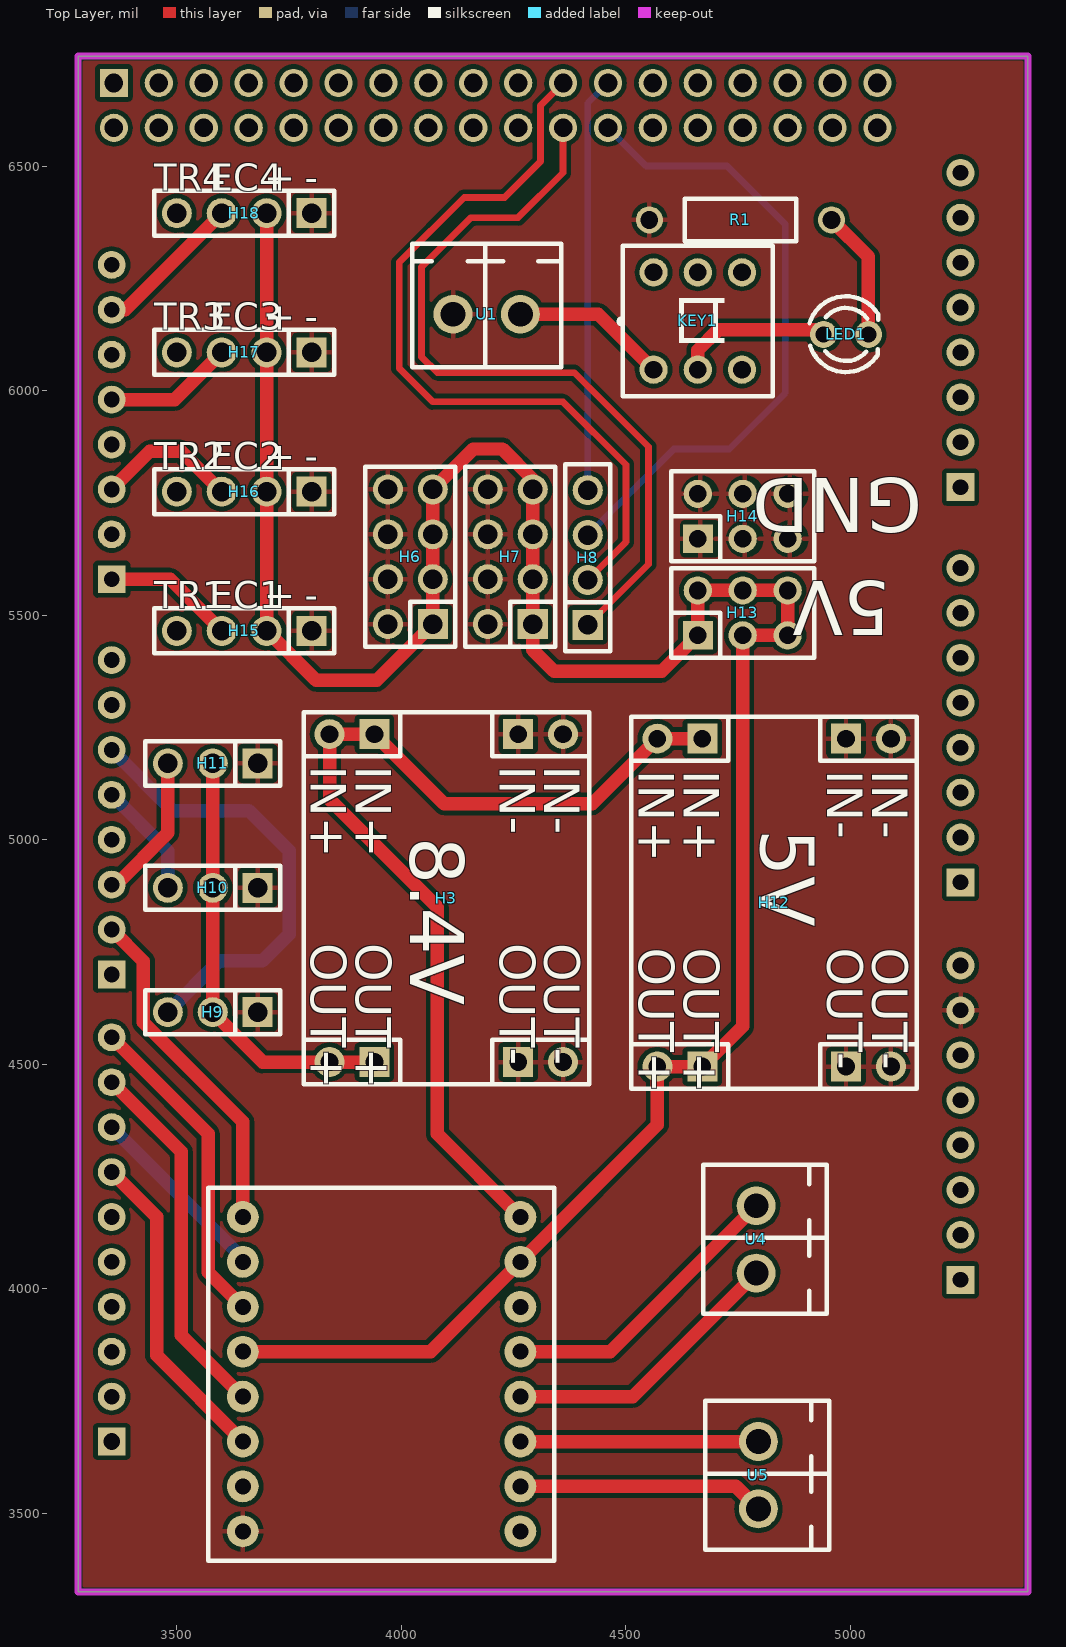
[diagram p0: Top Layer view]
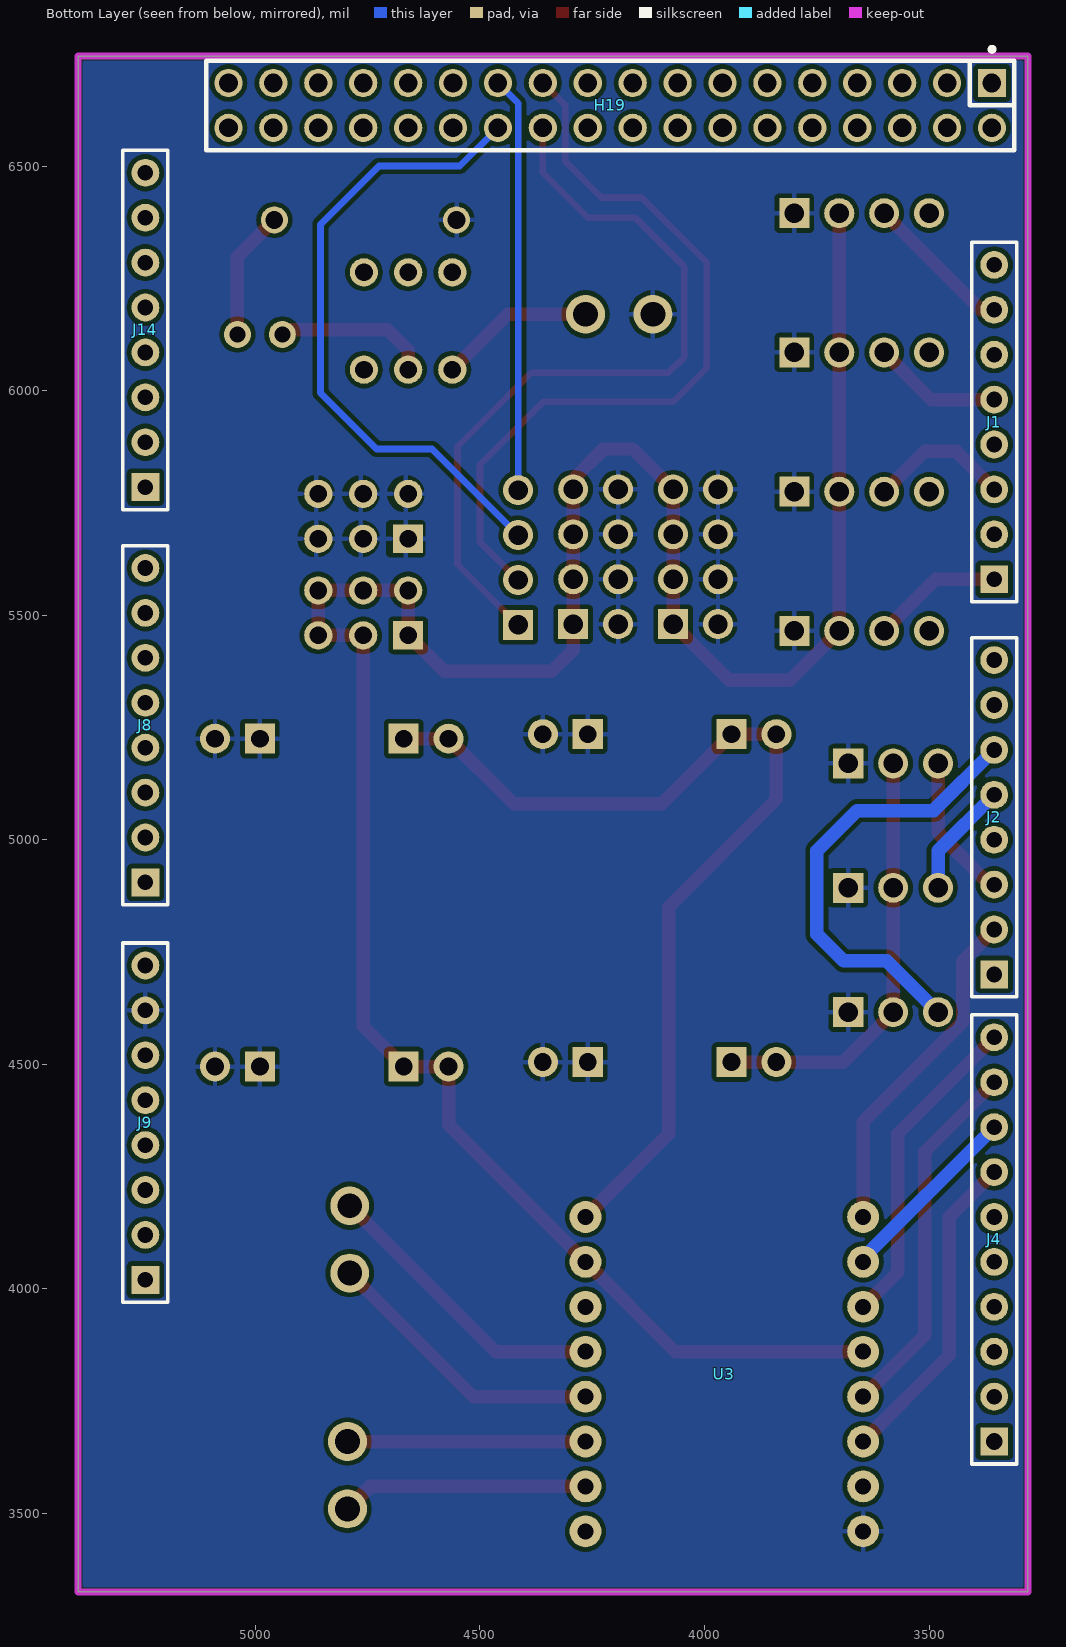
[diagram p1: Bottom Layer view, seen from below]
# Altium PCB MISC49940.pcbdoc
Units mil, origin at the board's own origin, x right, y up, seen from the top; angles counter-clockwise.
Board outline 2115 x 3420 mil, 2 copper layers (Top Layer, Bottom Layer), stack 62.206 mil thick; 28 components, 38 nets, 191 pads, 0 vias.

## Layer stack, top to bottom
Top Solder Mask Layer: solder mask 0.394, Dk 3.3
Top Layer: signal copper 1.379
Dielectric1: surface 59.449, FR4, Dk 4.5
Bottom Layer: signal copper 1.378
Bottom Solder Mask Layer: solder mask 0.394, Dk 3.3

## Board outline
3280,6745 3280,3325 5395,3325 5395,6745

## Design rules (kind name [scope] priority, off if disabled: settings)
BoardOutlineClearance copperThickness2oz_1 [All] p2 off: genericclearance=7.99 ignorepadtopadclearanceinfootprint=FALSE except(0: Arc-SplitContinuation Track-SplitContinuation SMDPad-SplitContinuation THPad-SplitContinuation Via-SplitContinuation Fill-SplitContinuation Region-SplitContinuation Poly-SplitContinuation Text-SplitContinuation Hole-SplitContinuation; 5.98: Arc-CutoutEdge Track-CutoutEdge SMDPad-CutoutEdge THPad-CutoutEdge Via-CutoutEdge Text-CutoutEdge; 6.9: Hole-OutlineEdge Hole-CutoutEdge; 10: Poly-OutlineEdge Poly-CutoutEdge; 11.81: Arc-OutlineEdge Track-OutlineEdge SMDPad-OutlineEdge THPad-OutlineEdge Via-OutlineEdge Fill-OutlineEdge Region-OutlineEdge Text-OutlineEdge Fill-CutoutEdge Region-CutoutEdge)
BoardOutlineClearance Plane_innerPlane_1 [All] p4 off: genericclearance=4.02 ignorepadtopadclearanceinfootprint=FALSE except(0: Arc-SplitContinuation Track-SplitContinuation SMDPad-SplitContinuation THPad-SplitContinuation Via-SplitContinuation Fill-SplitContinuation Region-SplitContinuation Poly-SplitContinuation Text-SplitContinuation Hole-SplitContinuation; 5.98: Arc-CutoutEdge Track-CutoutEdge SMDPad-CutoutEdge THPad-CutoutEdge Via-CutoutEdge Text-CutoutEdge; 6.9: Hole-OutlineEdge Hole-CutoutEdge; 10: Poly-OutlineEdge Poly-CutoutEdge; 11.81: Arc-OutlineEdge Track-OutlineEdge SMDPad-OutlineEdge THPad-OutlineEdge Via-OutlineEdge Fill-OutlineEdge Region-OutlineEdge Text-OutlineEdge Fill-CutoutEdge Region-CutoutEdge)
BoardOutlineClearance Copper_copperRegion_1 [All] p6 off: genericclearance=4.02 ignorepadtopadclearanceinfootprint=FALSE except(0: Arc-SplitContinuation Track-SplitContinuation SMDPad-SplitContinuation THPad-SplitContinuation Via-SplitContinuation Fill-SplitContinuation Region-SplitContinuation Poly-SplitContinuation Text-SplitContinuation Hole-SplitContinuation; 5.98: Arc-CutoutEdge Track-CutoutEdge SMDPad-CutoutEdge THPad-CutoutEdge Via-CutoutEdge Text-CutoutEdge; 6.9: Hole-OutlineEdge Hole-CutoutEdge; 10: Poly-OutlineEdge Poly-CutoutEdge; 11.81: Arc-OutlineEdge Track-OutlineEdge SMDPad-OutlineEdge THPad-OutlineEdge Via-OutlineEdge Fill-OutlineEdge Region-OutlineEdge Text-OutlineEdge Fill-CutoutEdge Region-CutoutEdge)
BoardOutlineClearance copperThickness1oz_1 [All] p8: genericclearance=4.02 ignorepadtopadclearanceinfootprint=FALSE except(0: Arc-SplitContinuation Track-SplitContinuation SMDPad-SplitContinuation THPad-SplitContinuation Via-SplitContinuation Fill-SplitContinuation Region-SplitContinuation Poly-SplitContinuation Text-SplitContinuation Hole-SplitContinuation; 5.98: Arc-CutoutEdge Track-CutoutEdge SMDPad-CutoutEdge THPad-CutoutEdge Via-CutoutEdge Text-CutoutEdge; 6.9: Hole-OutlineEdge Hole-CutoutEdge; 10: Poly-OutlineEdge Poly-CutoutEdge; 11.81: Arc-OutlineEdge Track-OutlineEdge SMDPad-OutlineEdge THPad-OutlineEdge Via-OutlineEdge Fill-OutlineEdge Region-OutlineEdge Text-OutlineEdge Fill-CutoutEdge Region-CutoutEdge)
Clearance copperThickness2oz [All] p1 off: gap=7.99 ignorepadtopadclearanceinfootprint=FALSE except(5.98: SMDPad-Track SMDPad-SMDPad THPad-Track SMDPad-THPad THPad-THPad Track-Via SMDPad-Via THPad-Via Via-Via Fill-SMDPad Region-SMDPad Fill-THPad Region-THPad Fill-Via Region-Via Fill-Fill Fill-Region Region-Region Arc-Track Arc-SMDPad Arc-THPad Arc-Via Fill-Arc Region-Arc Arc-Arc Text-Track SMDPad-Text Text-THPad Text-Via Fill-Text Region-Text Arc-Text Text-Text; 6.9: Hole-Track Hole-SMDPad Hole-THPad Hole-Via Fill-Hole Region-Hole Hole-Arc Hole-Text; 10: Poly-Track Poly-SMDPad Poly-THPad Poly-Via Poly-Fill Poly-Region Poly-Poly Poly-Arc Poly-Text Poly-Hole; 11.81: Fill-Track Region-Track)
Clearance Plane_innerPlane [All] p3 off: gap=4.02 ignorepadtopadclearanceinfootprint=FALSE except(5.98: SMDPad-Track SMDPad-SMDPad THPad-Track SMDPad-THPad THPad-THPad Track-Via SMDPad-Via THPad-Via Via-Via Fill-SMDPad Region-SMDPad Fill-THPad Region-THPad Fill-Via Region-Via Fill-Fill Fill-Region Region-Region Arc-Track Arc-SMDPad Arc-THPad Arc-Via Fill-Arc Region-Arc Arc-Arc Text-Track SMDPad-Text Text-THPad Text-Via Fill-Text Region-Text Arc-Text Text-Text; 6.9: Hole-Track Hole-SMDPad Hole-THPad Hole-Via Fill-Hole Region-Hole Hole-Arc Hole-Text; 10: Poly-Track Poly-SMDPad Poly-THPad Poly-Via Poly-Fill Poly-Region Poly-Poly Poly-Arc Poly-Text Poly-Hole; 11.81: Fill-Track Region-Track)
Clearance Copper_copperRegion [All] p5 off: gap=4.02 ignorepadtopadclearanceinfootprint=FALSE except(5.98: SMDPad-Track SMDPad-SMDPad THPad-Track SMDPad-THPad THPad-THPad Track-Via SMDPad-Via THPad-Via Via-Via Fill-SMDPad Region-SMDPad Fill-THPad Region-THPad Fill-Via Region-Via Fill-Fill Fill-Region Region-Region Arc-Track Arc-SMDPad Arc-THPad Arc-Via Fill-Arc Region-Arc Arc-Arc Text-Track SMDPad-Text Text-THPad Text-Via Fill-Text Region-Text Arc-Text Text-Text; 6.9: Hole-Track Hole-SMDPad Hole-THPad Hole-Via Fill-Hole Region-Hole Hole-Arc Hole-Text; 10: Poly-Track Poly-SMDPad Poly-THPad Poly-Via Poly-Fill Poly-Region Poly-Poly Poly-Arc Poly-Text Poly-Hole; 11.81: Fill-Track Region-Track)
Clearance copperThickness1oz [All] p7: gap=4.02 ignorepadtopadclearanceinfootprint=FALSE except(5.98: SMDPad-Track SMDPad-SMDPad THPad-Track SMDPad-THPad THPad-THPad Track-Via SMDPad-Via THPad-Via Via-Via Fill-SMDPad Region-SMDPad Fill-THPad Region-THPad Fill-Via Region-Via Fill-Fill Fill-Region Region-Region Arc-Track Arc-SMDPad Arc-THPad Arc-Via Fill-Arc Region-Arc Arc-Arc Text-Track SMDPad-Text Text-THPad Text-Via Fill-Text Region-Text Arc-Text Text-Text; 6.9: Hole-Track Hole-SMDPad Hole-THPad Hole-Via Fill-Hole Region-Hole Hole-Arc Hole-Text; 10: Poly-Track Poly-SMDPad Poly-THPad Poly-Via Poly-Fill Poly-Region Poly-Poly Poly-Arc Poly-Text Poly-Hole; 11.81: Fill-Track Region-Track)
DiffPairsRouting differentialPair [All] p1: maxlimit=6 minlimit=6 mostfreqgap=6 toplayer_minwidth=5 toplayer_prefwidth=10 toplayer_maxwidth=100 toplayer_mingap=6 toplayer_prefgap=6 toplayer_maxgap=6 bottomlayer_minwidth=5 bottomlayer_prefwidth=10 bottomlayer_maxwidth=100 bottomlayer_mingap=6 bottomlayer_prefgap=6 bottomlayer_maxgap=6 maxuncoupledlength=10
HoleToHoleClearance otherClearance [All] p1: gap=11.81 allowstackedmicrovias=TRUE
Length netLength [All] p1: minlimit=0 maxlimit=0
PasteMaskExpansion pasteMaskExpansion [All] p1: expansion=0
PlaneConnect innerPlane [All] p1: planeconnectstyle=Relief reliefexpansion=20 reliefentries=4 reliefconductorwidth=10 reliefairgap=10
PolygonConnect copperRegion [All] p1: connectstyle=Relief reliefconductorwidth=10 reliefentries=4 polygonreliefangle="90 Angle" airgapwidth=10 via.connectstyle=Relief via.reliefconductorwidth=10 via.reliefentries=4 via.polygonreliefangle="90 Angle" via.airgapwidth=10
RoutingVias viaSize [All] p1: holewidth=12.01 width=24.02 viastyle="Through Hole" minholewidth=11.81 minwidth=19.68 maxholewidth=248.03 maxwidth=393.7
SolderMaskExpansion solderMaskExpansion [IsVia] p1: expansion=-1000 istentingtop=TRUE
SolderMaskExpansion solderMaskExpansion [All] p2: expansion=2 istentingtop=FALSE
Width copperThickness2oz_2 [All] p1 off: maxlimit=100 minlimit=8 preferedwidth=10
Width copperThickness1oz_2 [All] p2: maxlimit=100 minlimit=5 preferedwidth=10

## Components (designator, comment, footprint, x,y, rotation, side; value= is the part's Value field where it differs from the comment)
H3 "" HDR-TH_8P-P2.54-V-M 4360,5235 r270 top
H6 "" HDR-TH_8P-P2.54-V-M-R2-C4-S2.54 4020,5630 r90 top
H7 "" HDR-TH_8P-P2.54-V-M-R2-C4-S2.54 4242.5,5630 r90 top
H8 "" HDR-TH_4P-P2.54-V-F 4415,5628.27 r90 top
H9 "" HDR-TH_3P-P2.54-V-M 3580,4616.01 r180 top
H10 "" HDR-TH_3P-P2.54-V-M 3580,4892.9 r180 top
H11 "" HDR-TH_3P-P2.54-V-M 3580,5169.79 r180 top
H12 "" HDR-TH_8P-P2.54-V-M 5090,5225 r270 top
H13 "" HDR-TH_6P-P2.54-V-F-R2-C3-S2.54 4760,5505 r0 top
H14 "" HDR-TH_6P-P2.54-V-F-R2-C3-S2.54 4760,5720 r0 top
H15 "" HDR-TH_4P-P2.54-V-M 3650,5465 r180 top
H16 "" HDR-TH_4P-P2.54-V-M 3650,5775 r180 top
H17 "" HDR-TH_4P-P2.54-V-M 3650,6085 r180 top
H18 "" HDR-TH_4P-P2.54-V-M 3650,6395 r180 top
H19 "X6521WV-2×18H-C30D60" HDR-TH_36P-2.54-V-M-R2-C18-S2.54 4210,6635 r0 bottom
J1 "3-way TX/RX" HDR-M-2.54_1X8 3355,5980 r90 bottom
J2 "PWM D2~D7" HDR-M-2.54_1X8 3355,5100 r90 bottom
J4 "PWM_D8~D13" HDR-M-2.54_1X10 3355,4110 r90 bottom
J8 "HDR-M-2.54_1x8" HDR-M-2.54_1X8 5245,5305 r90 bottom
J9 "HDR-M-2.54_1x8" HDR-M-2.54_1X8 5245,4420 r90 bottom
J14 "HDR-M-2.54_1x8" HDR-M-2.54_1X8 5245,6185 r90 bottom
KEY1 "Self-locking switch" SW-TH_6P-L8.5-W8.5-P2.54 4660,6155 r0 top
LED1 "" LED_TH-3mm 4990,6125 r0 top
R1 "1kΩ" Res_1/4W 4755,6380 r180 top
U1 "2P-P3.81_KF2EDGV-3.81-2P" CONN-TH_2P-P3.81_KF2EDGV-3.81-2P 4190,6170 r180 top
U3 "" tb6612 4265,4160 r180 bottom
U4 "2P-P3.81_KF2EDGV-3.81-2P" CONN-TH_2P-P3.81_KF2EDGV-3.81-2P 4790,4110 r90 top
U5 "2P-P3.81_KF2EDGV-3.81-2P" CONN-TH_2P-P3.81_KF2EDGV-3.81-2P 4795,3585 r90 top

## Footprints (in the part's own frame and the unit in brackets; to place one, negate y for a bottom-side part, rotate by r counter-clockwise, add the part's x,y. Pads: shape width x height; smd on the part's side, far side on the other; paste and mask are expansions set on the pad)
CONN-TH_2P-P3.81_KF2EDGV-3.81-2P [mm]
  round 2.2 hole 1.4: 1(-1.905,0) 2(1.905,0)
  silkscreen extent -4.21,-4 4.21,3
HDR-M-2.54_1X8 [mil]
  rect 62x62 hole 35: 1(-400,0)
  round 62 hole 35: 2(-300,0) 3(-200,0) 4(-100,0) 5(0,0) 6(100,0) 7(200,0) 8(300,0)
  silkscreen extent -450,-50 350,50
HDR-M-2.54_1X10 [mil]
  rect 62x62 hole 37.2: 1(-450,0)
  round 62 hole 35: 2(-350,0) 3(-250,0) 4(-150,0) 5(-50,0) 6(50,0) 7(150,0) 8(250,0) 9(350,0) 10(450,0)
  silkscreen extent -500,-50 500,50
HDR-TH_3P-P2.54-V-M [mm]
  rect 1.7x1.7 hole 1.1: 1(-2.54,0)
  round 1.7 hole 1.1: 2(0,0) 3(2.54,0)
  silkscreen extent -3.81,-1.25 3.81,1.25
HDR-TH_4P-P2.54-V-F [mm]
  rect 1.7x1.7 hole 1.1: 1(-3.81,0)
  round 1.7 hole 1.1: 2(-1.27,0) 3(1.27,0) 4(3.81,0)
  silkscreen extent -5.29,-1.27 5.29,1.27
HDR-TH_4P-P2.54-V-M [mm]
  rect 1.7x1.7 hole 1.1: 1(-3.81,0)
  round 1.7 hole 1.1: 2(-1.27,0) 3(1.27,0) 4(3.81,0)
  silkscreen extent -5.08,-1.27 5.08,1.27
HDR-TH_6P-P2.54-V-F-R2-C3-S2.54 [mm]
  rect 1.7x1.6 hole 1: 1(-2.54,-1.27)
  round 1.6 hole 1: 2(-2.54,1.27) 3(0,-1.27) 4(0,1.27) 5(2.54,-1.27) 6(2.54,1.27)
  silkscreen extent -4.04,-2.54 4.04,2.54
HDR-TH_8P-P2.54-V-M [mm]
  round 1.7 hole 1: 1(0,0) 4(0,-13.208) 5(18.542,0) 8(18.542,-13.208)
  rect 1.7x1.7 hole 1: 2(0,-2.54) 3(0,-10.668) 6(18.542,-2.54) 7(18.542,-10.668)
  silkscreen extent -1.25,-14.68 19.79,1.47
HDR-TH_8P-P2.54-V-M-R2-C4-S2.54 [mm]
  rect 1.7x1.7 hole 1.1: 1(-3.81,-1.27)
  round 1.7 hole 1.1: 2(-3.81,1.27) 3(-1.27,-1.27) 4(-1.27,1.27) 5(1.27,-1.27) 6(1.27,1.27) 7(3.81,-1.27) 8(3.81,1.27)
  silkscreen extent -5.08,-2.54 5.08,2.54
HDR-TH_36P-2.54-V-M-R2-C18-S2.54 [mm]
  rect 1.6x1.6 hole 1.05: 1(-21.59,-1.27)
  round 1.6 hole 1.05: 2(-21.59,1.27) 3(-19.05,-1.27) 4(-19.05,1.27) 5(-16.51,-1.27) 6(-16.51,1.27) 7(-13.97,-1.27) 8(-13.97,1.27) 9(-11.43,-1.27) 10(-11.43,1.27) 11(-8.89,-1.27) 12(-8.89,1.27) 13(-6.35,-1.27) 14(-6.35,1.27) 15(-3.81,-1.27) 16(-3.81,1.27) 17(-1.27,-1.27) 18(-1.27,1.27) 19(1.27,-1.27) 20(1.27,1.27) 21(3.81,-1.27) 22(3.81,1.27) 23(6.35,-1.27) 24(6.35,1.27) 25(8.89,-1.27) 26(8.89,1.27) 27(11.43,-1.27) 28(11.43,1.27) 29(13.97,-1.27) 30(13.97,1.27) 31(16.51,-1.27) 32(16.51,1.27) 33(19.05,-1.27) 34(19.05,1.27) 35(21.59,-1.27) 36(21.59,1.27)
  silkscreen extent -22.86,-3.3 22.86,2.54
LED_TH-3mm [mil]
  round 60 hole 36 paste+0 mask+2: 1(-50,0) 2(50,0)
  silkscreen extent -81,-84 72,85
Res_1/4W [mil]
  round 60 hole 39.37 paste+0 mask+2: 1(-202.76,0) 2(202.76,0)
  silkscreen extent -124,-47 124,47
SW-TH_6P-L8.5-W8.5-P2.54 [mm]
  round 1.6 hole 1: 1(-2.5,-2.75) 2(0,-2.75) 3(2.5,-2.75) 4(-2.5,2.75) 5(0,2.75) 6(2.5,2.75)
  silkscreen extent -4.47,-4.25 4.25,4.25
tb6612 [mm]
  round 1.8 hole 0.9: 1(0,0) 2(0,-2.54) 3(0,-5.08) 4(0,-7.62) 5(0,-10.16) 6(0,-12.7) 7(0,-15.24) 8(0,-17.78) 9(15.697,-17.78) 10(15.697,-15.24) 11(15.697,-12.7) 12(15.697,-10.16) 13(15.697,-7.62) 14(15.697,-5.08) 15(15.697,-2.54) 16(15.697,0)

## Nets (pads, with @x,y where several pads share a name; then routed paths per layer and width w, separated by ;. In a path a pad name is that pad's centre, name@x,y a point inside that pad or via, vN(x,y) a via of type N, cw(c..) or ccw(c..) an arc to the next point about the centre after c; other vN are vias at no path point)
5V: H6.1 H6.3 H6.5 H6.7 H7.1 H7.3 H7.5 H7.7 H12.7 H12.8 H13.1 H13.2 H13.3 H13.4 H13.5 H13.6 H15.2 H16.2 H17.2 H18.2 U3.2 U3.13 | length 5644.8
  Top Layer w30: U3.13 4065,3860 U3.2 4570,4365 H12.8 H12.7 4760,4585 H13.3 H13.5 H13.6 H13.4 H13.2 H13.1 4580,5375 4340,5375 4292.5,5422.5 H7.1 H7.3 H7.5 H7.7 4292.5,5802.5 4225,5870 4160,5870 H6.7 H6.5 H6.3 H6.1 3945,5355 3810,5355 H15.2 H16.2 H17.2 H18.2
8.4V: H3.7 H3.8 H9.2 H10.2 H11.2 | length 959.8
  Top Layer w30: H11.2 H10.2 H9.2 3691.01,4505 H3.8 H3.7
8.5V: J9.8
12V: KEY1.2 LED1.1 | length 346.1
  Top Layer w30: KEY1.2 4659.99,6089.99 4705,6135 4930,6135 LED1.1
$1N513: LED1.2 R1.1 | length 289.1
  Top Layer w30: R1.1 5040,6297.76 LED1.2
$1N515: KEY1.1 U1.1 | length 347.6
  Top Layer w30: U1.1 4438.31,6170 KEY1.1
AIN1: J4.10 U3.14 | length 721
  Top Layer w30: J4.10 3570,4345 3570,4037 U3.14
AIN2: J4.8 U3.15 | length 421
  Bottom Layer w30: J4.8 3647,4068 U3.15
AO1: U3.4 U4.2 | length 659.6
  Top Layer w30: U3.4 4465,3860 U4.2
AO2: U3.5 U4.1 | length 638.9
  Top Layer w30: U3.5 4515,3760 U4.1
BIN1: J4.9 U3.12 | length 821
  Top Layer w30: J4.9 3510,4305 3510,3897 U3.12
BIN2: J4.7 U3.11 | length 721
  Top Layer w30: J4.7 3455,4160 3455,3852 U3.11
BO1: U3.7 U5.1 | length 550.7
  Top Layer w30: U3.7 4745,3560 U5.1
BO2: U3.6 U5.2 | length 530
  Top Layer w30: U3.6 U5.2
ECHO1: H15.3 J1.1 | length 292.6
  Top Layer w30: J1.1 3485,5580 H15.3
ECHO2: H16.3 J1.3 | length 317.5
  Top Layer w30: J1.3 3440,5865 3510,5865 H16.3
ECHO3: H17.3 J1.5 | length 288.5
  Top Layer w30: J1.5 3495,5980 H17.3
ECHO4: H18.3 J1.7 | length 334.1
  Top Layer w30: J1.7 3385,6180 H18.3
GND: H3.1 H3.2 H3.5 H3.6 H6.2 H6.4 H6.6 H6.8 H7.2 H7.4 H7.6 H7.8 H9.1 H10.1 H11.1 H12.1 H12.2 H12.5 H12.6 H14.1 H14.2 H14.3 H14.4 H14.5 H14.6 H15.1 H16.1 H17.1 H18.1 J9.7 R1.2 U1.2 U3.9
PWM8: J2.1
PWMA: J2.2 U3.16 | length 761
  Top Layer w30: J2.2 3425.55,4729.45 3425.55,4593.46 3647,4372.01 U3.16
PWMB: U3.10
R1: H8.1 H19.22 | length 1742.5
  Top Layer w15: H19.22 4360,6485 4260,6385 4155,6385 4045,6275 4045,6075 4080,6040 4385,6040 4550,5875 4550,5613.27 H8.1
R2: H8.2 H19.21 | length 1724.9
  Top Layer w15: H19.21 4310,6635 4310,6510 4230,6430 4140,6430 3995,6285 3995,6050 4070,5975 4360,5975 4500,5835 4500,5663.27 H8.2
R3: H8.3 H19.24 | length 1430.3
  Bottom Layer w15: H8.3 4606.73,5870 4730,5870 4855,5995 4855,6370 4725,6500 4545,6500 H19.24
R4: H8.4 H19.23 | length 925.4
  Bottom Layer w15: H8.4 4415,6640 H19.23
S1: H9.3 J2.6 | length 1015.3
  Bottom Layer w30: J2.6 3490,5065 3660,5065 3750,4975 3750,4790 3690,4730 3593.99,4730 H9.3
S2: H10.3 J2.5 | length 258.9
  Bottom Layer w30: J2.5 3480,4975 H10.3
S3: H11.3 J2.3 | length 327.4
  Top Layer w30: J2.3 3365,4900 3480,5015 H11.3
TRIG1: H15.4
TRIG2: H16.4
TRIG3: H17.4
TRIG4: H18.4
TWIG1: J1.2
TWIG2: J1.4
TWIG3: J1.6
TWIG4: J1.8
VCC: H3.3 H3.4 H12.3 H12.4 U3.1 | length 2205.3
  Top Layer w30: U3.1 4080,4345 4080,4850 3840,5090 H3.4 H3.3 4095,5080 4425,5080 H12.4 H12.3
pads on no net: H19.1 H19.2 H19.3 H19.4 H19.5 H19.6 H19.7 H19.8 H19.9 H19.10 H19.11 H19.12 H19.13 H19.14 H19.15 H19.16 H19.17 H19.18 H19.19 H19.20 H19.25 H19.26 H19.27 H19.28 H19.29 H19.30 H19.31 H19.32 H19.33 H19.34 H19.35 H19.36 J2.4 J2.7 J2.8 J4.1 J4.2 J4.3 J4.4 J4.5 J4.6 J8.1 J8.2 J8.3 J8.4 J8.5 J8.6 J8.7 J8.8 J9.1 J9.2 J9.3 J9.4 J9.5 J9.6 J14.1 J14.2 J14.3 J14.4 J14.5 J14.6 J14.7 J14.8 KEY1.3 KEY1.4 KEY1.5 KEY1.6 U3.3 U3.8

## Polygon pours and split planes (outlines as drawn)
GND on Top Layer (solid, remove dead copper, pour order 0): 3000,7015 3000,3000 5790,3000 5790,7015
GND on Bottom Layer (solid, remove dead copper, pour order 2): 3010,6985 3010,3105 5625,3105 5625,6985

## Keep-outs
Board Outline Layer:
  the board outline again, w15

## Silkscreen, mask and mechanical layers (free items; w line width, h text height)
Top Silkscreen Layer:
  text "TR4" at 3450,6445 h60
  text "EC4" at 3572.83,6445 h60
  text "+" at 3695,6445 h60
  text "-" at 3785,6445 h60
  text "TR3" at 3450,6135 h60
  text "EC3" at 3572.83,6135 h60
  text "+" at 3695,6135 h60
  text "-" at 3785,6135 h60
  text "TR2" at 3450,5825 h60
  text "EC2" at 3572.83,5825 h60
  text "+" at 3695,5825 h60
  text "-" at 3785,5825 h60
  text "GND" at 5160,5805 h120 r180
  text "5V" at 5088.9,5575 h120 r180
  text "TR1" at 3450,5515 h60
  text "EC1" at 3572.83,5515 h60
  text "+" at 3695,5515 h60
  text "-" at 3785,5515 h60
  text "5V" at 4800,5023.45 h120 r270
  text "8.4V" at 4020,5005 h120 r270